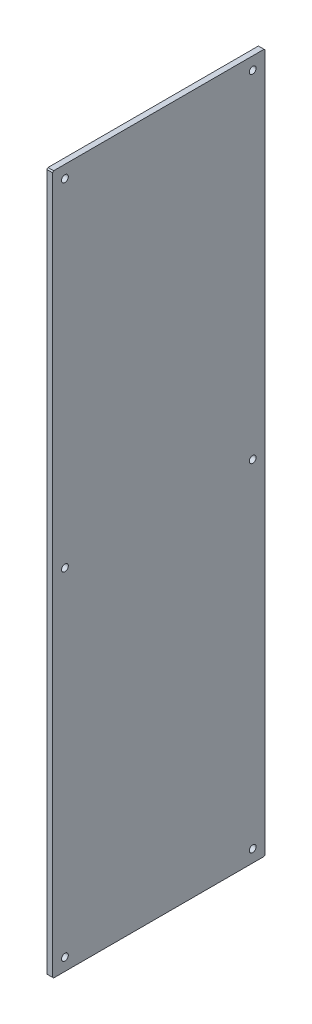
SolidWorks part; units mm, degrees
material "PC(透明)"
ref_plane "前基準面" through (0, 0, 0) normal (0, 0, 1) x (1, 0, 0)
ref_plane "上基準面" through (0, 0, 0) normal (0, 1, 0) x (1, 0, 0)
ref_plane "右基準面" through (0, 0, 0) normal (1, 0, 0) x (0, 0, -1)
sketch "草图1" plane through (0, 0, 0) normal (1, 0, 0) x (0, 0, -1)
  line L1 (94, 309) -> (-94, 309)
  line L2 (94, 309) -> (94, -309)
  line L3 (94, -309) -> (-94, -309)
  line L4 (-94, 309) -> (-94, -309)
  line L5 (94, 309) -> (-94, -309) construction
  line L6 (94, -309) -> (-94, 309) construction
  point P0 (0, 0)
  dimension "D1" = 188
  dimension "D2" = 618
extrude "凸台-拉伸1" add sketch "草图1" along normal blind 5
chamfer "倒角1" distance 1 angle 45 4 edges at (2.5, -309, -94) (2.5, -309, 94) (2.5, 309, -94) (2.5, 309, 94)
sketch "草图2" plane through (0, 0, 0) normal (-1, 0, 0) x (0, 0, 1)
  line L0 (-94, -308) -> (-94, 308) construction
  line L1 (-93, 309) -> (93, 309) construction
  line L2 (58.8862, 0) -> (0, 0) construction
  line L3 (0, 0) -> (0, 69.8386) construction
  line L5 (83, -298) -> (-83, -298) construction
  line L6 (83, -298) -> (83, 298) construction
  line L7 (83, 298) -> (-83, 298) construction
  line L8 (-83, -298) -> (-83, 298) construction
  line L9 (83, -298) -> (-83, 298) construction
  line L10 (83, 298) -> (-83, -298) construction
  circle A0 centre (-83, 298) radius 3
  circle A1 centre (-83, -298) radius 3
  circle A2 centre (83, -298) radius 3
  circle A3 centre (83, 298) radius 3
  circle A8 centre (83, 0) radius 3
  circle A9 centre (-83, 0) radius 3
  dimension "D1" = 6
  dimension "D2" = 11
  dimension "D3" = 11
extrude "切除-拉伸1" cut sketch "草图2" against normal through all
sketch "草图3" plane through (5, 0, 0) normal (1, 0, 0) x (0, 0, -1)
  line L0 (-74, -249) -> (-94, -249) construction
  line L2 (-74, -259) -> (-94, -259)
  line L3 (-74, -239) -> (-94, -239)
  line L4 (-93, -309) -> (93, -309) construction
  line L5 (-94, 308) -> (-94, -308) construction
  arc A0 (-74, -259) -> (-74, -239) centre (-74, -249) ccw
  arc A1 (-94, -239) -> (-94, -259) centre (-94, -249) ccw
  point P4 (-84, -249)
  dimension "D1" = 20
  dimension "D2" = 60
  dimension "D3" = 20
